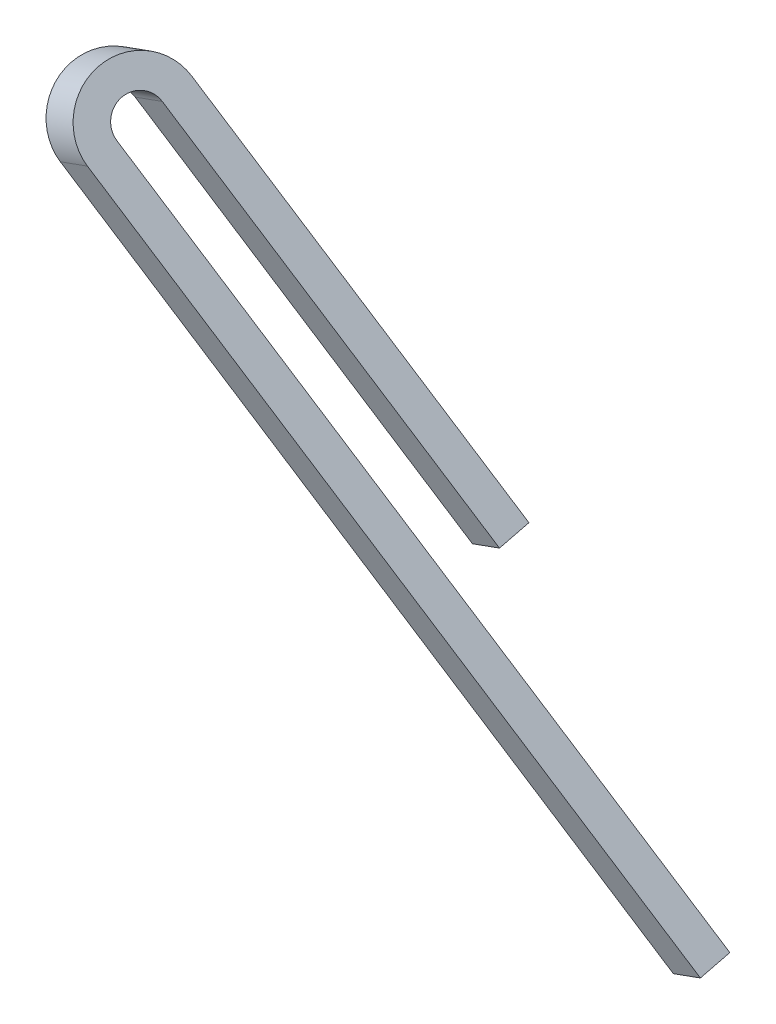
SolidWorks part; units mm, degrees
ref_plane "前视基准面" through (0, 0, 0) normal (0, 0, 1) x (1, 0, 0)
ref_plane "上视基准面" through (0, 0, 0) normal (0, 1, 0) x (1, 0, 0)
ref_plane "右视基准面" through (0, 0, 0) normal (1, 0, 0) x (0, 0, -1)
sketch "草图2" plane through (290.97, -860.871, 2246.0116) normal (0.8091, 0.4948, 0.317) x (-0.1246, -0.3828, 0.9154)
  line L0 (0, 712.5) -> (0, -209.4279)
  line L1 (0, 712.5) -> (0, -712.5) construction
  line L2 (-124, 297.7587) -> (-124, -209.4279)
  line L3 (-124, 137.7587) -> (-124, 227.7587) construction
  arc A0 (-124, -209.4279) -> (0, -209.4279) centre (-62, -209.4279) ccw
extrude "拉伸-薄壁1" add sketch "草图2" against normal mid plane 68 thin
